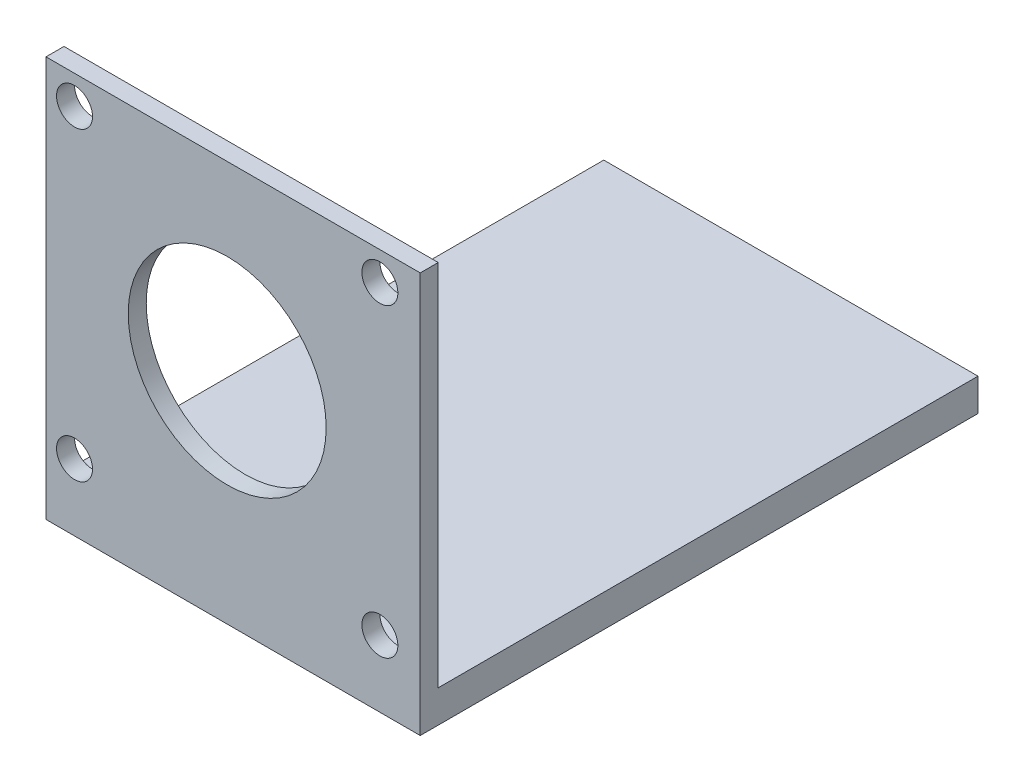
from build123d import *

# Parameters (mm, degrees)
EXTRUDE_1_DEPTH          = 5
SKETCH_4_R               = 27.5
CUT_EXTRUDE_4_DEPTH      = 20
SKETCH_5_W               = 104
SKETCH_5_H               = 9
EXTRUDE_2_DEPTH          = 150
CUT_EXTRUDE_5_DEPTH      = 171.582117426
CUT_EXTRUDE_5_DEPTH_BACK = 171.582117426
SKETCH_6_R               = 5


with BuildPart() as part:
    # 草图1 → 凸台-拉伸1 (new body)
    with BuildSketch(Plane.XY):
        Polygon((-50.354639151, -47.265777393), (-50.354639151, -53.645360849), (-50.354639151, -60.995360849), (53.645360849, -60.995360849), (53.645360849, -53.645360849), (53.645360849, 50.354639151), (-50.354639151, 50.354639151), align=None)
    extrude(amount=EXTRUDE_1_DEPTH)

    # 草图4 → 切除-拉伸4 (cut)
    with BuildSketch(Plane.XY.offset(5)):
        Circle(SKETCH_4_R)
    extrude(amount=-CUT_EXTRUDE_4_DEPTH, mode=Mode.SUBTRACT)

    # 草图5 → 凸台-拉伸2 (add)
    with BuildSketch(Plane(origin=(0, 0, 0), x_dir=(-1, 0, 0), z_dir=(0, 0, -1))):
        with Locations((-1.645360849, -56.495360849)):
            Rectangle(SKETCH_5_W, SKETCH_5_H)
    extrude(amount=EXTRUDE_2_DEPTH)

    # 草图6 → 切除-拉伸5 (cut, two sides: drawn at the far end of the back side and taken through both)
    with BuildSketch(Plane(origin=(0, 0, 0), x_dir=(-1, 0, 0), z_dir=(0, 0, -1)).offset(-CUT_EXTRUDE_5_DEPTH_BACK)):
        with Locations((-42.426406871, 42.426406871)):
            Circle(SKETCH_6_R)
        with Locations((42.426406871, 42.426406871)):
            Circle(SKETCH_6_R)
        with Locations((42.426406871, -42.426406871)):
            Circle(SKETCH_6_R)
        with Locations((-42.426406871, -42.426406871)):
            Circle(SKETCH_6_R)
    extrude(amount=CUT_EXTRUDE_5_DEPTH + CUT_EXTRUDE_5_DEPTH_BACK, mode=Mode.SUBTRACT)


solid = part.part
